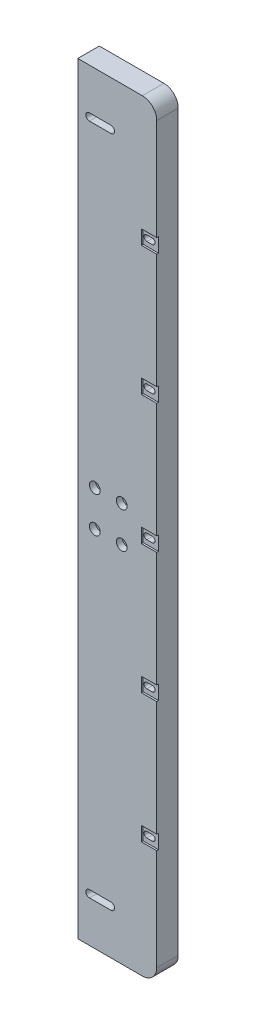
from build123d import *

# Parameters (mm, degrees)
SKETCH_1_W                = 44
SKETCH_1_H                = 425
EXTRUDE_1_DEPTH           = 12
FILLET_1_R                = 8
CUT_EXTRUDE_1_DEPTH       = 6
CUT_EXTRUDE_2_DEPTH       = 214.972544968
SKETCH_5_W                = 8.5
SKETCH_5_H                = 8
CUT_EXTRUDE_3_DEPTH       = 1
CUT_EXTRUDE_4_DEPTH       = 4
CUT_EXTRUDE_5_DEPTH       = 214.785523364
PATTERN_LINEAR_1_COUNT    = 5
PATTERN_LINEAR_1_PITCH    = 72
HOLE_WIZARD_1_D           = 3.4
HOLE_WIZARD_1_CBORE_D     = 6
HOLE_WIZARD_1_CBORE_DEPTH = 3.4


with BuildPart() as part:
    # 草图1 → 凸台-拉伸1 (new body)
    with BuildSketch(Plane.XY):
        Rectangle(SKETCH_1_W, SKETCH_1_H)
    extrude(amount=EXTRUDE_1_DEPTH)

    # 圆角1
    fillet_1_edges = [part.edges().sort_by_distance(p)[0] for p in [
        (22, 212.5, 6),
        (22, -212.5, 6),
    ]]
    fillet(fillet_1_edges, radius=FILLET_1_R)

    # 草图3 → 切除-拉伸1 (cut)
    with BuildSketch(Plane(origin=(0, 0, 0), x_dir=(-1, 0, 0), z_dir=(0, 0, -1))):
        with BuildLine():
            Line((15.5, 183.5), (3.5, 183.5))
            ThreePointArc((3.5, 183.5), (-0.5, 187.5), (3.5, 191.5))
            Line((3.5, 191.5), (15.5, 191.5))
            ThreePointArc((15.5, 191.5), (19.5, 187.5), (15.5, 183.5))
        make_face()
        with BuildLine():
            Line((15.5, -183.5), (3.5, -183.5))
            ThreePointArc((3.5, -183.5), (-0.5, -187.5), (3.5, -191.5))
            Line((3.5, -191.5), (15.5, -191.5))
            ThreePointArc((15.5, -191.5), (19.5, -187.5), (15.5, -183.5))
        make_face()
    extrude(amount=-CUT_EXTRUDE_1_DEPTH, mode=Mode.SUBTRACT)

    # 草图4 → 切除-拉伸2 (cut, through all)
    with BuildSketch(Plane(origin=(0, 0, 0), x_dir=(-1, 0, 0), z_dir=(0, 0, -1))):
        with BuildLine():
            Line((3.5, 189.5), (15.5, 189.5))
            ThreePointArc((15.5, 189.5), (17.5, 187.5), (15.5, 185.5))
            Line((15.5, 185.5), (3.5, 185.5))
            ThreePointArc((3.5, 185.5), (1.5, 187.5), (3.5, 189.5))
        make_face()
        with BuildLine():
            Line((3.5, -189.5), (15.5, -189.5))
            ThreePointArc((15.5, -189.5), (17.5, -187.5), (15.5, -185.5))
            Line((15.5, -185.5), (3.5, -185.5))
            ThreePointArc((3.5, -185.5), (1.5, -187.5), (3.5, -189.5))
        make_face()
    extrude(amount=-CUT_EXTRUDE_2_DEPTH, mode=Mode.SUBTRACT)

    # 草图5 → 切除-拉伸3 (cut)
    with BuildSketch(Plane.XY.offset(12)):
        with Locations((17.75, 144)):
            Rectangle(SKETCH_5_W, SKETCH_5_H)
        with Locations((17.75, 72)):
            Rectangle(SKETCH_5_W, SKETCH_5_H)
        with Locations((17.75, 0)):
            Rectangle(SKETCH_5_W, SKETCH_5_H)
        with Locations((17.75, -72)):
            Rectangle(SKETCH_5_W, SKETCH_5_H)
        with Locations((17.75, -144)):
            Rectangle(SKETCH_5_W, SKETCH_5_H)
    extrude(amount=-CUT_EXTRUDE_3_DEPTH, mode=Mode.SUBTRACT)

    # 草图6 → 切除-拉伸4 (cut)
    with BuildSketch(Plane(origin=(0, 0, 0), x_dir=(-1, 0, 0), z_dir=(0, 0, -1))):
        with BuildLine():
            Line((-18.5, 147), (-15.5, 147))
            ThreePointArc((-15.5, 147), (-12.5, 144), (-15.5, 141))
            Line((-15.5, 141), (-18.5, 141))
            ThreePointArc((-18.5, 141), (-21.5, 144), (-18.5, 147))
        make_face()
    cut_extrude_4 = extrude(amount=-CUT_EXTRUDE_4_DEPTH, mode=Mode.SUBTRACT)

    # 草图7 → 切除-拉伸5 (cut, through all)
    with BuildSketch(Plane(origin=(0, 0, 4), x_dir=(-1, 0, 0), z_dir=(0, 0, -1))):
        with BuildLine():
            Line((-18.5, 145.6), (-15.5, 145.6))
            ThreePointArc((-15.5, 145.6), (-13.9, 144), (-15.5, 142.4))
            Line((-15.5, 142.4), (-18.5, 142.4))
            ThreePointArc((-18.5, 142.4), (-20.1, 144), (-18.5, 145.6))
        make_face()
    cut_extrude_5 = extrude(amount=-CUT_EXTRUDE_5_DEPTH, mode=Mode.SUBTRACT)

    # 阵列(线性)1: 切除-拉伸4, 切除-拉伸5 ×5
    with Locations(*[(0, -i * PATTERN_LINEAR_1_PITCH, 0) for i in range(1, PATTERN_LINEAR_1_COUNT)]):
        add(cut_extrude_4, mode=Mode.SUBTRACT)
        add(cut_extrude_5, mode=Mode.SUBTRACT)

    # 打孔尺寸根据内六角圆柱头螺钉的类型1 (through all)
    with Locations(Plane.XY.offset(12)):
        with Locations((2.5, 10), (-12.5, 10), (2.5, -10), (-12.5, -10)):
            CounterBoreHole(HOLE_WIZARD_1_D / 2, HOLE_WIZARD_1_CBORE_D / 2, HOLE_WIZARD_1_CBORE_DEPTH)


solid = part.part
